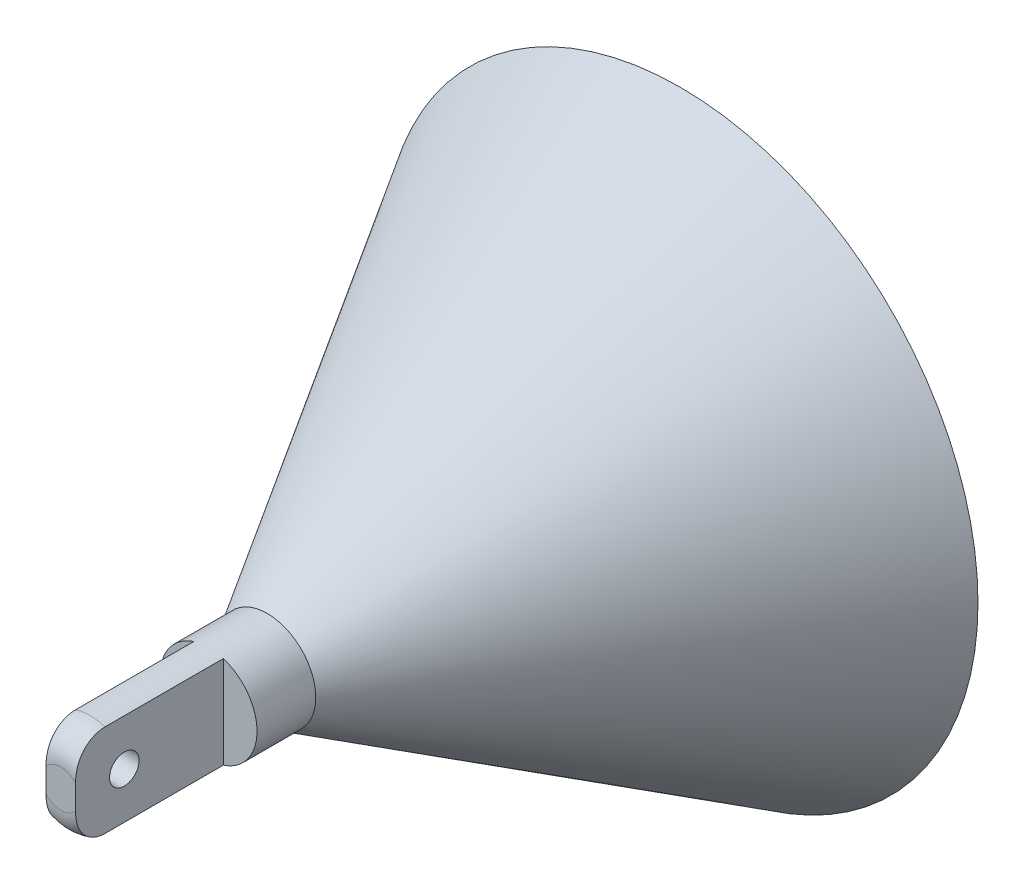
from build123d import *

# Parameters (mm, degrees)
SKETCH2_W          = 22.958469665
SKETCH2_H          = 42.577525561
CUT_EXTRUDE1_DEPTH = 50
SKETCH3_R          = 5
CUT_EXTRUDE2_DEPTH = 50
FILLET1_R          = 10


with BuildPart() as part:
    # Sketch1 → Revolve1 (revolve)
    with BuildSketch(Plane(origin=(0, 0, 0), x_dir=(1, 0, 0), z_dir=(0, 1, 0)), mode=Mode.PRIVATE) as revolve1_sk:
        Polygon((0, 0), (16.40283031, 0), (16.40283031, 69.874110237), (100.714201253, 209.625997087), (8.201415155, 209.625997087), (0, 209.625997087), align=None)
    revolve(revolve1_sk.sketch.rotate(Axis((0, 0, 0), (0, 0, -1)), 180), axis=Axis((0, 0, 0), (0, 0, -1)))

    # Sketch2 → Cut-Extrude1 (cut)
    with BuildSketch(Plane.XY):
        with Locations((-16.479234833, -2.283064826)):
            Rectangle(SKETCH2_W, SKETCH2_H)
        with Locations((16.479234833, -2.283064826)):
            Rectangle(SKETCH2_W, SKETCH2_H)
    extrude(amount=-CUT_EXTRUDE1_DEPTH, mode=Mode.SUBTRACT)

    # Sketch3 → Cut-Extrude2 (cut)
    with BuildSketch(Plane(origin=(5, 0, 0), x_dir=(0, 0, -1), z_dir=(1, 0, 0))):
        with Locations(Location((16.498374342, 0, 0), (0, 0, 90))):
            Circle(SKETCH3_R)
    extrude(amount=-CUT_EXTRUDE2_DEPTH, mode=Mode.SUBTRACT)

    # Fillet1
    fillet1_edges = [part.edges().sort_by_distance(p)[0] for p in [
        (0, -16.40283031, 0),
        (0, 16.40283031, 0),
    ]]
    fillet(fillet1_edges, radius=FILLET1_R)

    # Sketch4 → Cut-Revolve1 (revolve, cut)
    with BuildSketch(Plane(origin=(0, 0, 0), x_dir=(0, 0, -1), z_dir=(1, 0, 0)), mode=Mode.PRIVATE) as cut_revolve1_sk:
        Polygon((77.000967597, 14.066660466), (233.165313112, 99.181638622), (233.165313112, 0), (77.000967597, 0), align=None)
    revolve(cut_revolve1_sk.sketch.rotate(Axis((0, 0, -233.165313112), (0, 0, 1)), 197.747662393), axis=Axis((0, 0, -233.165313112), (0, 0, 1)), mode=Mode.SUBTRACT)


solid = part.part
